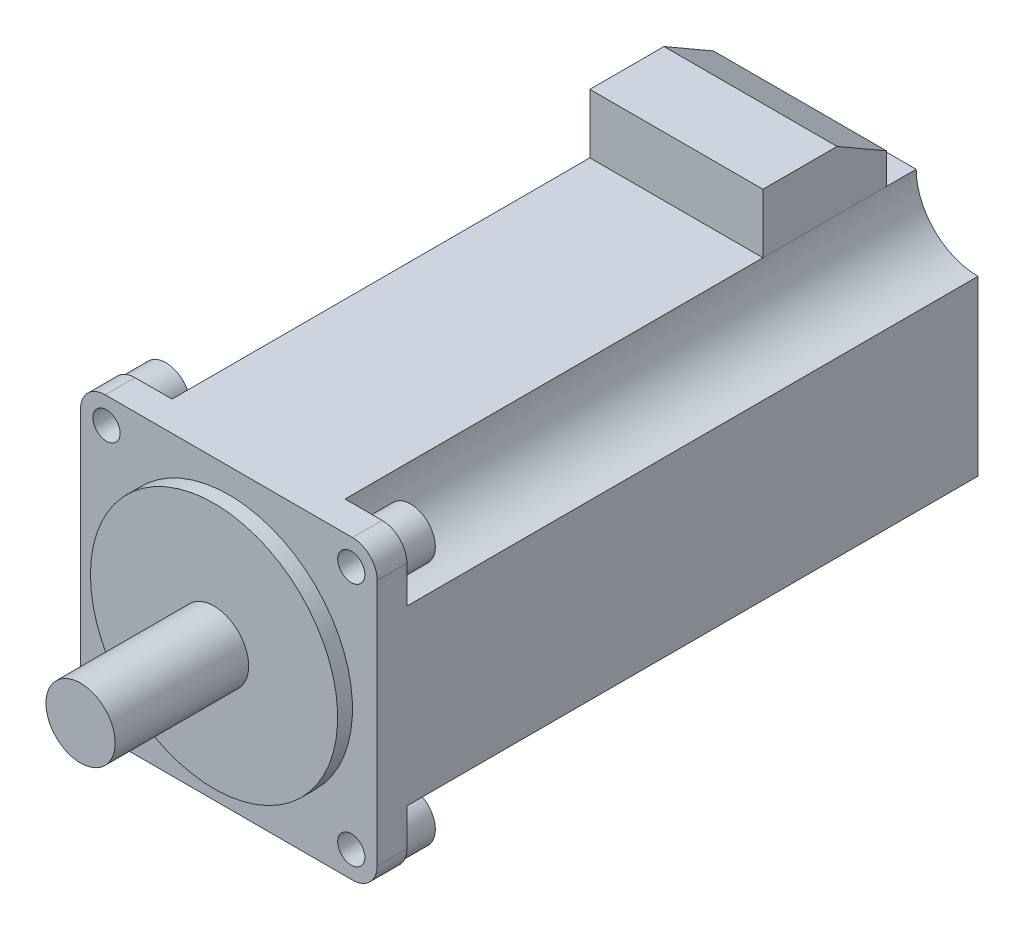
SolidWorks part; units mm, degrees
material "S45C"
ref_plane "Front Plane" through (0, 0, 0) normal (0, 0, 1) x (1, 0, 0)
ref_plane "Top Plane" through (0, 0, 0) normal (0, 1, 0) x (1, 0, 0)
ref_plane "Right Plane" through (0, 0, 0) normal (1, 0, 0) x (0, 0, -1)
sketch "Sketch1" plane through (0, 0, 0) normal (0, 0, 1) x (1, 0, 0)
  circle A0 centre (0, 0) radius 7
  dimension "D1" = 14
extrude "Boss-Extrude1" add sketch "Sketch1" against normal blind 30
sketch "Sketch2" plane through (0, 0, -30) normal (0, 0, -1) x (-1, 0, 0)
  circle A0 centre (0, 0) radius 25
  dimension "D1" = 50
extrude "Boss-Extrude2" add sketch "Sketch2" against normal blind 3
sketch "Sketch3" plane through (0, 0, -30) normal (0, 0, -1) x (-1, 0, 0)
  line L1 (-30, 30) -> (30, 30)
  line L2 (-30, 30) -> (-30, -30)
  line L3 (-30, -30) -> (30, -30)
  line L4 (30, 30) -> (30, -30)
  line L5 (-30, 30) -> (30, -30) construction
  line L6 (-30, -30) -> (30, 30) construction
  point P0 (0, 0)
  dimension "D1" = 60
  dimension "D2" = 60
extrude "Boss-Extrude3" add sketch "Sketch3" along normal blind 6
sketch "Sketch4" plane through (0, 0, -36) normal (0, 0, -1) x (-1, 0, 0)
  line L4 (30, -30) -> (30, 30)
  line L5 (30, 30) -> (-30, 30)
  line L6 (-30, 30) -> (-30, -30)
  line L7 (-30, -30) -> (30, -30)
  line L8 (30, -17.5) -> (30, 17.5)
  line L9 (17.5, 30) -> (-17.5, 30)
  line L10 (-30, 17.5) -> (-30, -17.5)
  line L11 (-17.5, -30) -> (17.5, -30)
  arc A0 (-30, 17.5) -> (-17.5, 30) centre (-30, 30) ccw
  arc A1 (17.5, 30) -> (30, 17.5) centre (30, 30) ccw
  arc A2 (-17.5, -30) -> (-30, -17.5) centre (-30, -30) ccw
  arc A3 (30, -17.5) -> (17.5, -30) centre (30, -30) ccw
  dimension "D2" = 25
  dimension "D1" = 0
extrude "Boss-Extrude4" add sketch "Sketch4" along normal blind 115.5
sketch "Sketch5" plane through (0, 30, 0) normal (0, 1, 0) x (1, 0, 0)
  line L0 (-17.5, 151.5) -> (-17.5, 36) construction
  line L1 (-17.5, 145.5) -> (17.5, 145.5)
  line L2 (-17.5, 145.5) -> (-17.5, 120.5)
  line L3 (-17.5, 120.5) -> (17.5, 120.5)
  line L4 (17.5, 145.5) -> (17.5, 120.5)
  line L5 (0, 0) -> (0, 156.2316) construction
  line L6 (-17.5, 151.5) -> (17.5, 151.5) construction
  dimension "D1" = 6
  dimension "D2" = 25
extrude "Boss-Extrude5" add sketch "Sketch5" along normal blind 12
chamfer "Chamfer1" distance 10 angle 30 1 edges at (0, 42, -145.5)
hole_wizard "Ø5.5 (5.5) Diameter Hole1" positions "Sketch7" profile "Sketch6" hole size "Ø5.5" standard "Iso"
sketch "Sketch7" plane through (0, 0, -30) normal (0, 0, 1) x (1, 0, 0)
  line L0 (0, 48.7057) -> (0, 0) construction
  line L1 (0, 0) -> (24.7487, 24.7487) construction
  line L3 (0, 0) -> (57.255, 0) construction
  circle A0 centre (0, 0) radius 35 construction
  point P0 (24.7487, 24.7487)
  point P18 (-24.7487, 24.7487)
  point P20 (24.7487, -24.7487)
  point P21 (-24.7487, -24.7487)
  dimension "D1" = 70
  dimension "D2" = 45
sketch "Sketch6" plane through (24.7487, 24.7487, -30) normal (1, 0, 0) x (0, -1, 0)
  line L0 (0, 0) -> (0, 21.6524)
  line L1 (0, 21.6524) -> (2.75, 20)
  line L2 (2.75, 20) -> (2.75, 0)
  line L5 (2.75, 0) -> (0, 0)
  line L10 (0, 21.6524) -> (-2.75, 20) construction
  line L11 (0, -6.35) -> (0, 107.95) construction
  dimension "孔直径" = 5.5
  dimension "孔深度" = 20
  dimension "导头角度" = 118
fillet "Fillet1" radius 5 4 edges at (30, -30, -33) (-30, -30, -33) (-30, 30, -33) (30, 30, -33)
sketch "Sketch8" plane through (0, 0, -36) normal (0, 0, -1) x (-1, 0, 0)
  circle A0 centre (-24.7487, 24.7487) radius 5
  circle A1 centre (-24.7487, -24.7487) radius 5
  circle A2 centre (24.7487, -24.7487) radius 5
  circle A3 centre (24.7487, 24.7487) radius 5
  dimension "D1" = 10
extrude "Boss-Extrude6" add sketch "Sketch8" along normal blind 6
